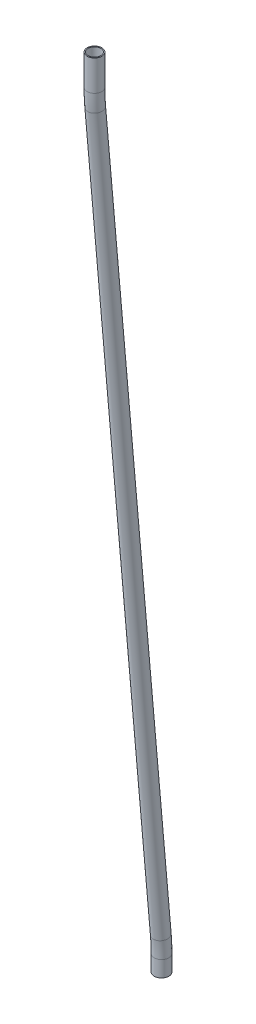
from build123d import *

# Parameters (mm, degrees)
SWEEP_THIN1_PROFILE_R   = 15
SWEEP_THIN1_PROFILE_R_2 = 13


with BuildPart() as part:
    # Sweep-Thin1: sweep along a curve in space
    with BuildLine() as sweep_thin1_path:
        Line((19403.083026604, -840, -3659.86490803), (19403.083026604, -807.464377163, -3659.86490803))
        ThreePointArc((19403.083026604, -807.464377163, -3659.86490803), (19403.083026604, -790.016622217, -3659.484196663), (19403.083026604, -772.602080064, -3658.342787267))
        Line((19403.083026604, -772.602080064, -3658.342787267), (19403.083026604, 756.627756068, -3524.552512679))
        ThreePointArc((19403.083026604, 756.627756068, -3524.552512679), (19403.083026604, 774.042298221, -3523.411103283), (19403.083026604, 791.490053167, -3523.030391916))
        Line((19403.083026604, 791.490053167, -3523.030391916), (19403.083026604, 854.025676004, -3523.030391916))
    # Sweep-Thin1 profile (on start of the path) → Sweep-Thin1 (sweep)
    with BuildSketch(Plane(origin=(19403.083026604, -840, -3659.86490803), x_dir=(0, 0, 1), z_dir=(0, 1, 0))):
        Circle(SWEEP_THIN1_PROFILE_R)
        Circle(SWEEP_THIN1_PROFILE_R_2, mode=Mode.SUBTRACT)
    sweep(path=sweep_thin1_path.line)


solid = part.part
